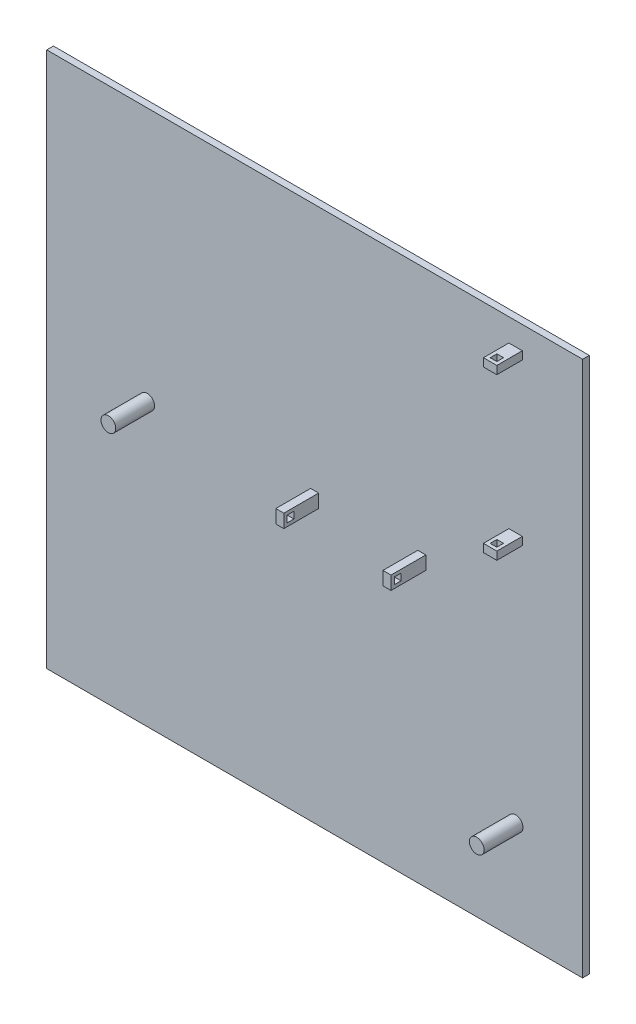
from build123d import *

# Parameters (mm, degrees)
SKETCH1_W               = 400
SKETCH1_H               = 400
SKETCH1_R               = 2.5
BOSS_EXTRUDE1_DEPTH     = 5
SKETCH4_R               = 5
CUT_EXTRUDE1_DEPTH      = 283.886903196
SKETCH6_W               = 6
SKETCH6_H               = 10
BOSS_EXTRUDE4_DEPTH     = 26
CUT_EXTRUDE2_DEPTH      = 348.922405142
CUT_EXTRUDE2_DEPTH_BACK = 348.922405142
SKETCH8_W               = 5
SKETCH8_H               = 5
SKETCH9_W               = 10
SKETCH9_H               = 6
BOSS_EXTRUDE5_DEPTH     = 19
CUT_EXTRUDE3_DEPTH      = 328.123829765
CUT_EXTRUDE3_DEPTH_BACK = 328.123829765
SKETCH10_W              = 5
SKETCH10_H              = 5
SKETCH11_R              = 5.5
BOSS_EXTRUDE7_DEPTH     = 29


with BuildPart() as part:
    # Sketch1 → Boss-Extrude1 (new body)
    with BuildSketch(Plane.XY):
        Rectangle(SKETCH1_W, SKETCH1_H)
        with Locations((0, 10)):
            Circle(SKETCH1_R, mode=Mode.SUBTRACT)
        with Locations((80, 10)):
            Circle(SKETCH1_R, mode=Mode.SUBTRACT)
        with Locations((150, 180)):
            Circle(SKETCH1_R, mode=Mode.SUBTRACT)
        with Locations((150, 60)):
            Circle(SKETCH1_R, mode=Mode.SUBTRACT)
    extrude(amount=BOSS_EXTRUDE1_DEPTH)

    # Sketch4 → Cut-Extrude1 (cut, through all)
    with BuildSketch(Plane.XY.offset(5)):
        with Locations((-125, 10)):
            Circle(SKETCH4_R)
        with Locations((150, -125)):
            Circle(SKETCH4_R)
    extrude(amount=-CUT_EXTRUDE1_DEPTH, mode=Mode.SUBTRACT)

    # Sketch6 → Boss-Extrude4 (add)
    with BuildSketch(Plane.XY.offset(5)):
        with Locations((0, 10)):
            Rectangle(SKETCH6_W, SKETCH6_H)
        with Locations((80, 10)):
            Rectangle(SKETCH6_W, SKETCH6_H)
    extrude(amount=BOSS_EXTRUDE4_DEPTH)

    # Sketch8 → Cut-Extrude2 (cut, two sides: drawn at the far end of the back side and taken through both)
    with BuildSketch(Plane(origin=(83, 0, 0), x_dir=(0, 0, -1), z_dir=(1, 0, 0)).offset(-CUT_EXTRUDE2_DEPTH_BACK)):
        with Locations((-26, 10)):
            Rectangle(SKETCH8_W, SKETCH8_H)
    extrude(amount=CUT_EXTRUDE2_DEPTH + CUT_EXTRUDE2_DEPTH_BACK, mode=Mode.SUBTRACT)

    # Sketch9 → Boss-Extrude5 (add)
    with BuildSketch(Plane.XY.offset(5)):
        with Locations((150, 180)):
            Rectangle(SKETCH9_W, SKETCH9_H)
        with Locations((150, 60)):
            Rectangle(SKETCH9_W, SKETCH9_H)
    extrude(amount=BOSS_EXTRUDE5_DEPTH)

    # Sketch10 → Cut-Extrude3 (cut, two sides: drawn at the far end of the back side and taken through both)
    with BuildSketch(Plane(origin=(0, 57, 0), x_dir=(-1, 0, 0), z_dir=(0, -1, 0)).offset(-CUT_EXTRUDE3_DEPTH_BACK)):
        with Locations((-150, -19)):
            Rectangle(SKETCH10_W, SKETCH10_H)
    extrude(amount=CUT_EXTRUDE3_DEPTH + CUT_EXTRUDE3_DEPTH_BACK, mode=Mode.SUBTRACT)

    # Sketch11 → Boss-Extrude7 (add)
    with BuildSketch(Plane.XY.offset(5)):
        with Locations((-125, 10)):
            Circle(SKETCH11_R)
        with Locations((150, -125)):
            Circle(SKETCH11_R)
    extrude(amount=BOSS_EXTRUDE7_DEPTH)


solid = part.part
